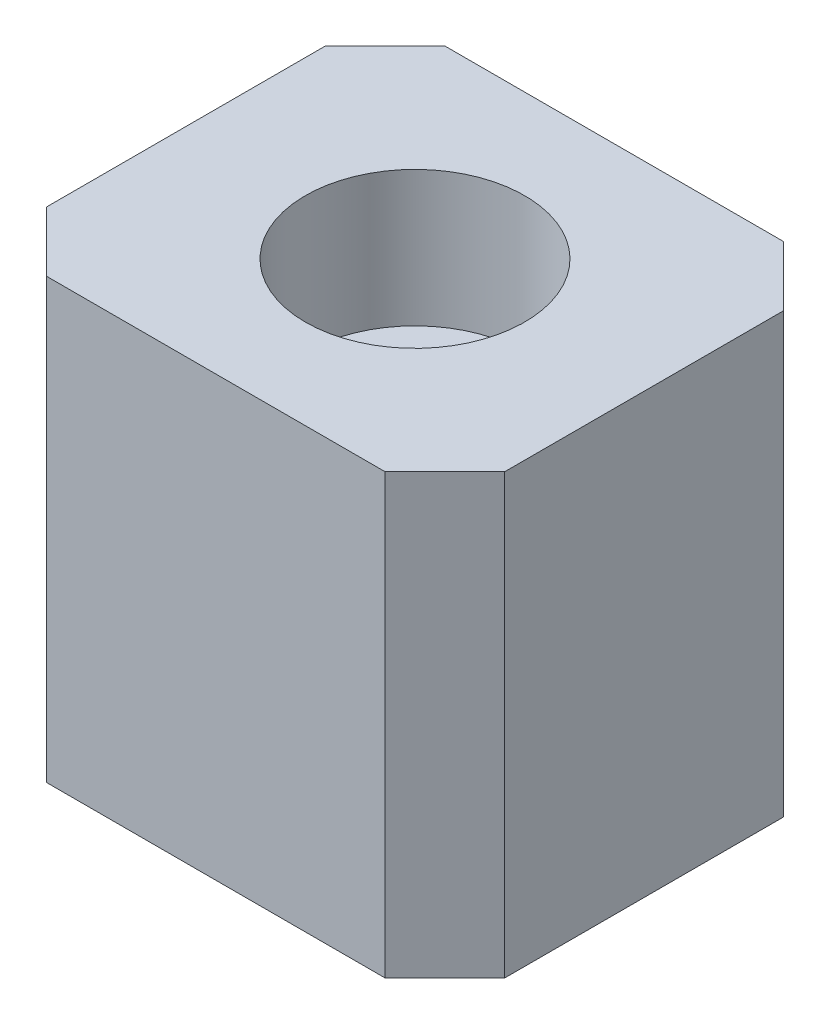
SolidWorks part; units mm, degrees
ref_plane "前视基准面" through (0, 0, 0) normal (0, 0, 1) x (1, 0, 0)
ref_plane "上视基准面" through (0, 0, 0) normal (0, 1, 0) x (1, 0, 0)
ref_plane "右视基准面" through (0, 0, 0) normal (1, 0, 0) x (0, 0, -1)
sketch "草图1" plane through (0, 0, 0) normal (0, 0, 1) x (1, 0, 0)
  line L1 (-11.5, 22) -> (11.5, 22)
  line L2 (-11.5, 22) -> (-11.5, 0)
  line L3 (-11.5, 0) -> (11.5, 0)
  line L4 (11.5, 22) -> (11.5, 0)
  dimension "D1" = 23
  dimension "D2" = 22
extrude "凸台-拉伸1" add sketch "草图1" along normal blind 20
hole_wizard "打孔尺寸(%根据)内六角圆柱头螺钉的类型1" positions "草图3" profile "草图2" counterbore size "M6" standard "GB" end condition through all
sketch "草图3" plane through (0, 22, 0) normal (0, 1, 0) x (1, 0, 0)
  line L0 (-11.5, -10) -> (11.5, -10) construction
  line L1 (-11.5, -20) -> (-11.5, 0) construction
  line L2 (11.5, -20) -> (11.5, 0) construction
  point P0 (0, -10)
sketch "草图2" plane through (0, 22, 10) normal (1, 0, 0) x (0, 0, 1)
  line L0 (0, 0) -> (0, 22)
  line L1 (0, 22) -> (3.3, 22)
  line L3 (3.3, 22) -> (3.3, 6.8)
  line L4 (3.3, 6.8) -> (5.5, 6.8)
  line L5 (5.5, 6.8) -> (5.5, 0)
  line L7 (5.5, 0) -> (0, 0)
  line L11 (0, -6.35) -> (0, 107.95) construction
  dimension "通孔孔直径" = 6.6
  dimension "通孔孔深度" = 22
  dimension "柱形沉头孔直径" = 11
  dimension "柱形沉头孔深度" = 6.8
chamfer "倒角1" distance 3 angle 45 4 edges at (-11.5, 11, 0) (-11.5, 11, 20) (11.5, 11, 20) (11.5, 11, 0)
